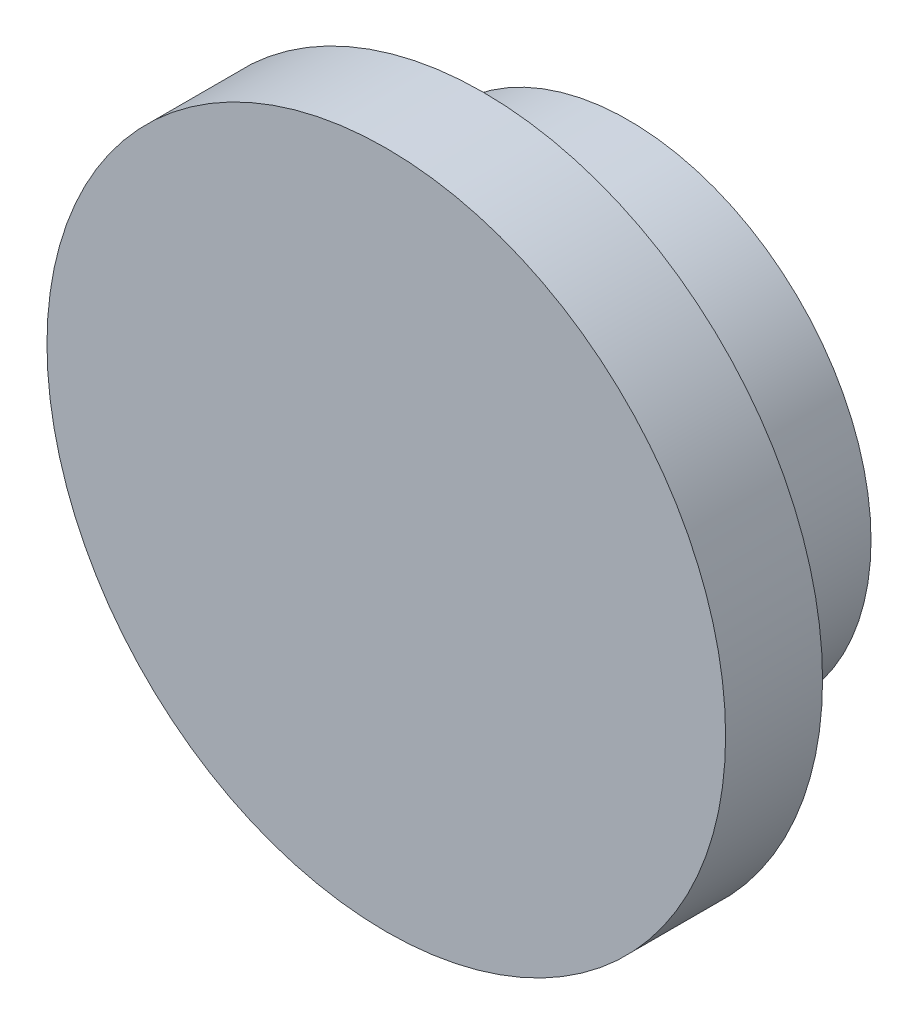
SolidWorks part; units mm, degrees
ref_plane "前视基准面" through (0, 0, 0) normal (0, 0, 1) x (1, 0, 0)
ref_plane "上视基准面" through (0, 0, 0) normal (0, 1, 0) x (1, 0, 0)
ref_plane "右视基准面" through (0, 0, 0) normal (1, 0, 0) x (0, 0, -1)
other "Configuration Table"
sketch "草图1" plane through (0, 0, 0) normal (0, 0, 1) x (1, 0, 0)
  circle A0 centre (0, 0) radius 5
  point P0 (0, 0)
  dimension "D1" = 10
extrude "凸台-拉伸1" add sketch "草图1" against normal blind 3
sketch "草图2" plane through (0, 0, 0) normal (0, 0, 1) x (1, 0, 0)
  circle A0 centre (0, 0) radius 7
  point P0 (0, 0)
  dimension "D1" = 14
extrude "凸台-拉伸2" add sketch "草图2" along normal blind 2
